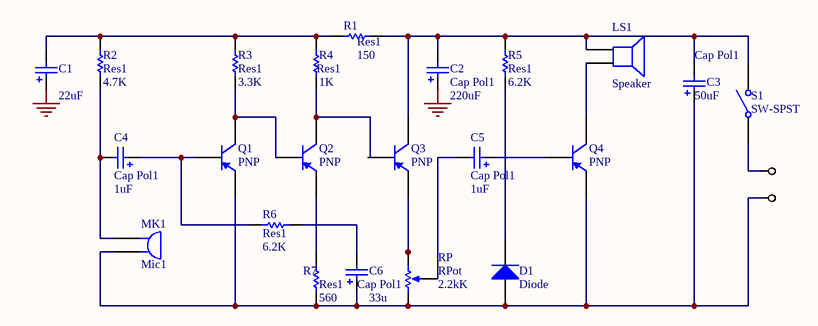
[diagram p0: MISC95146.SCHDOC]
# Altium project MISC95146.PRJPCB
1 sheet, 22 parts. Net scope: global (net labels, ports and power ports of the same name join across sheets).
Board files: MISC95146-6.PCBDOC, MISC95146.PCBDOC

## Sheet MISC95146.SCHDOC
size A4

### Parts
C1  value 22uF  [RB7.6-15]  (hidden comment: Cap Pol1)
C2  Cap Pol1  value 220uF  [RB7.6-15]
C3  Cap Pol1  value 50uF  [RB7.6-15]
C4  Cap Pol1  value 1uF  [RB7.6-15]
C5  Cap Pol1  value 1uF  [RB7.6-15]
C6  Cap Pol1  value 33u  [RB7.6-15]
D1  Diode  [DSO-C2/X3.3]
LS1  Speaker  [PIN2]
MK1  Mic1  [PIN2]
Q1  PNP  [SO-G3/C2.5]
Q2  PNP  [SO-G3/C2.5]
Q3  PNP  [SO-G3/C2.5]
Q4  PNP  [SO-G3/C2.5]
R1  Res1  value 150  [AXIAL-0.3]
R2  Res1  value 4.7K  [AXIAL-0.3]
R3  Res1  value 3.3K  [AXIAL-0.3]
R4  Res1  value 1K  [AXIAL-0.3]
R5  Res1  value 6.2K  [AXIAL-0.3]
R6  Res1  value 6.2K  [AXIAL-0.3]
R7  Res1  value 560  [AXIAL-0.3]
RP  RPot  value 2.2kK  [VR2]
S1  SW-SPST  [SPST-2]

### Nets
GND: C1.1 C2.1
NetC3_1: C3.1 C6.1 D1.1(A) MK1.2 Q1.3(E) Q4.3(E) R7.1 RP.1(TOP) S1.1(COMMON)
NetC1_2: C1.2 R1.1 R2.2 R3.2 R4.2
NetC2_2: C2.2 C3.2 LS1.1 Q3.1(C) R1.2 R5.2 S1.2(NO)
NetC4_1: C4.1 Q1.2(B) R6.2
NetC4_2: C4.2 MK1.1 R2.1
NetC5_1: C5.1 Q4.2(B)
NetC5_2: C5.2 RP.3(TAP)
NetC6_2: C6.2 R6.1
NetD1_2: D1.2(K) R5.1
NetLS1_2: LS1.2 Q4.1(C)
NetQ1_1: Q1.1(C) Q2.2(B) R3.1
NetQ2_1: Q2.1(C) R4.1
NetQ2_3: Q2.3(E) R7.2
NetQ3_3: Q3.3(E) RP.2(BOT)

Not connected (* = marked no-connect by the designer): Q3 2(B)

### Library data of the parts
C1-C6 = Cap Pol1: Polarized Capacitor (Radial); Published: 8-Jun-2000; Revision: July-2002: Re-released for DXP Platform.; Publisher: Altium Limited
D1 = Diode: Default Diode; Code - JEDEC: DO-214-AB; Published: 8-Jun-2000; Revision: July-2002: Re-released for DXP Platform.; Publisher: Altium Limited
LS1 = Speaker: Loudspeaker; Published: 24-Mar-1999; Revision: July-2002: Re-released for DXP Platform.; Publisher: Altium Limited
MK1 = Mic1: Microphone; Published: 24-Mar-1999; Revision: July-2002: Re-released for DXP Platform.; Publisher: Altium Limited
Q1-Q4 = PNP: PNP Bipolar Transistor; Code - JEDEC: SOT-23; Published: 8-Jun-2000; Revision: July-2002: Re-released for DXP Platform.; Publisher: Altium Limited
R1-R7 = Res1: Resistor; Published: 8-Jun-2000; Revision: July-2002: Re-released for DXP Platform.; Publisher: Altium Limited
RP = RPot: Potentiometer; Set Position: 0.5; Published: 8-Jun-2000; Revision: July-2002: Re-released for DXP Platform.; Publisher: Altium Limited
S1 = SW-SPST: Single-Pole, Single-Throw Switch; Published: 24-Mar-1999; Revision: July-2002: Re-released for DXP Platform.; Publisher: Altium Limited